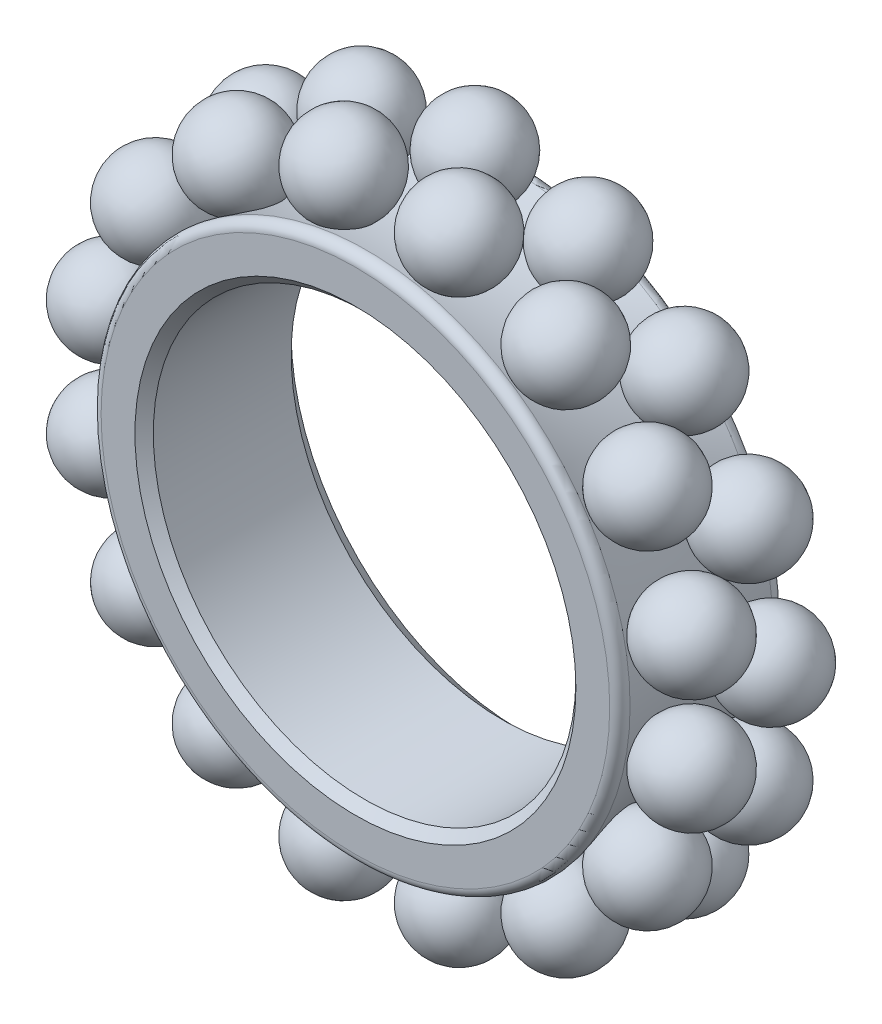
SolidWorks part; units mm, degrees
ref_plane "Front Plane" through (0, 0, 0) normal (0, 0, 1) x (1, 0, 0)
ref_plane "Top Plane" through (0, 0, 0) normal (0, 1, 0) x (1, 0, 0)
ref_plane "Right Plane" through (0, 0, 0) normal (1, 0, 0) x (0, 0, -1)
sketch "Sketch1" plane through (0, 0, 0) normal (0, 0, 1) x (1, 0, 0)
  circle A0 centre (0, 0) radius 29
  dimension "D1" = 58
extrude "Boss-Extrude1" add sketch "Sketch1" along normal mid plane 18
sketch "Sketch2" plane through (0, 0, 0) normal (0, 1, 0) x (1, 0, 0)
  line L0 (29, 9) -> (29, -9)
  line L1 (0, 0) -> (0, 17.246) construction
  line L2 (0, -9.9) -> (0, 9.9) construction
  arc A0 (29, 9) -> (29, -9) centre (58.6648, 0) ccw
revolve "Cut-Revolve1" cut sketch "Sketch2" angle 360 about L1
sketch "Sketch3" plane through (0, 0, 0) normal (0, 1, 0) x (1, 0, 0)
  line L0 (29, 9) -> (29, -9) construction
  line L1 (-36.5, -9) -> (36.5, -9) construction
  line L2 (-36.5, -9) -> (-36.5, 9)
  line L3 (-36.5, 9) -> (36.5, 9) construction
  line L4 (36.5, -9) -> (36.5, 9) construction
  line L5 (-36.5, -9) -> (36.5, 9) construction
  line L6 (-36.5, 9) -> (36.5, -9) construction
  line L7 (27.2087, 4) -> (37.2087, 4)
  arc A0 (36.5, 9) -> (36.5, -9) centre (-7.5908, 0) cw construction
  arc A1 (37.2087, 4) -> (27.2087, 4) centre (32.2087, 4) ccw
  point P0 (0, 0)
  dimension "D3" = 45
  dimension "D4" = 10
  dimension "D1" = 73
  dimension "D2" = 18
revolve "Revolve1" add sketch "Sketch3" angle 360 about L7
pattern_circular "CirPattern4" count 16 over 360 about axis through (0, 0, 0) along (0, 0, 1) of bodies 103
ref_plane "Plane1" through (0, 0, 0) normal (-0.5556, 0.8315, 0) x (0.8315, 0.5556, 0)
sketch "Sketch5" plane through (0, 0, 0) normal (-0.5556, 0.8315, 0) x (0.8315, 0.5556, 0)
  line L2 (0, -9) -> (0, 17.5869) construction
  line L3 (27.2087, -4) -> (37.2087, -4)
  line L4 (-36.5, -9) -> (36.5, -9) construction
  line L5 (-36.5, -9) -> (-36.5, 9) construction
  line L7 (36.5, -9) -> (36.5, 9) construction
  line L8 (-36.5, -9) -> (36.5, 9) construction
  line L9 (-36.5, 9) -> (36.5, -9) construction
  arc A0 (36.5, 9) -> (36.5, -9) centre (-7.5908, 0) cw construction
  arc A1 (27.2087, -4) -> (37.2087, -4) centre (32.2087, -4) ccw
  point P5 (0, 0)
  dimension "D3" = 45
  dimension "D4" = 10
  dimension "D1" = 73
  dimension "D2" = 18
revolve "Revolve2" add sketch "Sketch5" angle 360 about L3
pattern_circular "CirPattern5" count 16 over 360 about axis through (0, 0, 0) along (0, 0, 1) of bodies 119
sketch "Sketch6" plane through (0, 0, 9) normal (0, 0, 1) x (1, 0, 0)
  circle A0 centre (0, 0) radius 23
  dimension "D1" = 46
extrude "Cut-Extrude1" cut sketch "Sketch6" against normal through all
chamfer "Chamfer1" distance 1 angle 45 1 edges at (23, 0, 9)
chamfer "Chamfer2" distance 2 angle 45 1 edges at (23, 0, -9)
fillet "Fillet1" radius 1 2 edges at (29, 0, -9) (29, 0, 9)
